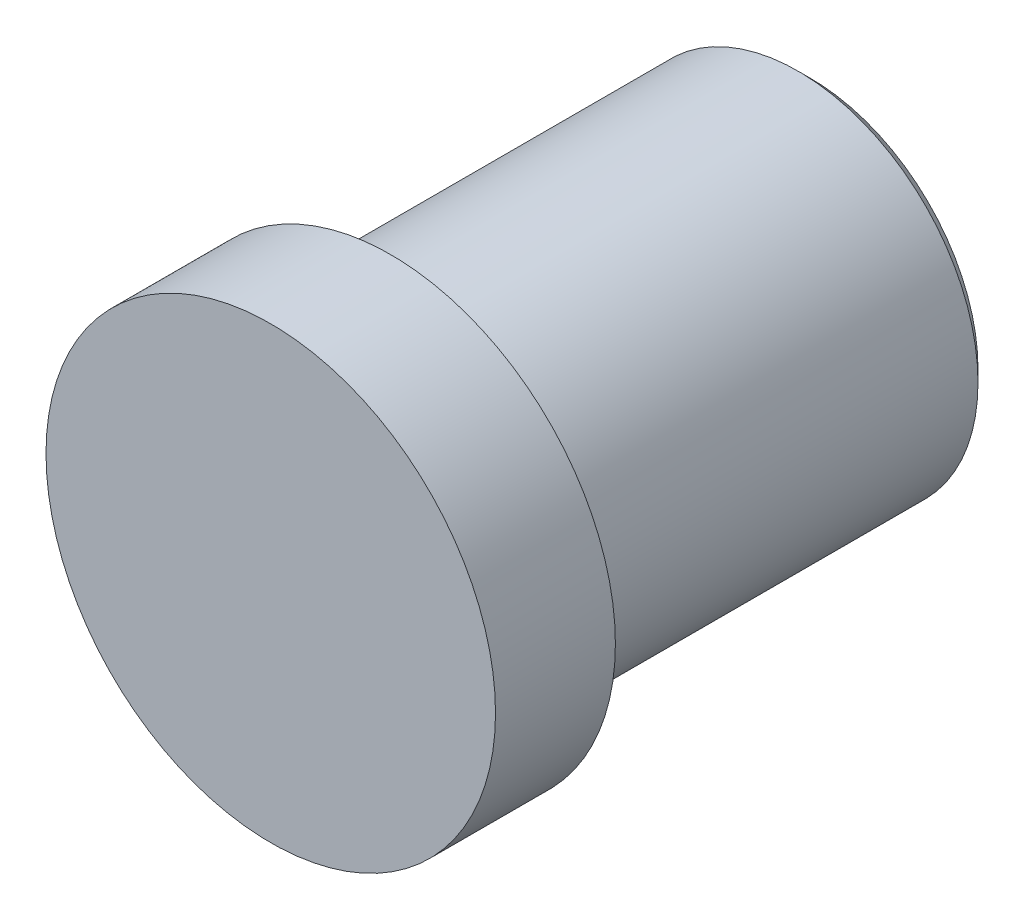
SolidWorks part; units mm, degrees
material "Q345"
ref_plane "前视基准面" through (0, 0, 0) normal (0, 0, 1) x (1, 0, 0)
ref_plane "上视基准面" through (0, 0, 0) normal (0, 1, 0) x (1, 0, 0)
ref_plane "右视基准面" through (0, 0, 0) normal (1, 0, 0) x (0, 0, -1)
sketch "草图1" plane through (0, 0, 0) normal (0, 0, 1) x (1, 0, 0)
  circle A0 centre (0, 0) radius 30
  circle A1 centre (0, 0) radius 20 construction
  dimension "D1" = 60
  dimension "D2" = 40
extrude "凸台-拉伸1" add sketch "草图1" along normal blind 70
sketch "草图2" plane through (0, 0, 70) normal (0, 0, 1) x (1, 0, 0)
  circle A0 centre (0, 0) radius 37.5
  dimension "D1" = 75
extrude "凸台-拉伸2" add sketch "草图2" along normal blind 20
chamfer "倒角2" distance 2 angle 45 1 edges at (30, 0, 0)
ref_axis "基准轴1" through (0, 0, 70) along (0, 0, -1)
sketch "草图3" plane through (0, 0, 0) normal (0, 1, 0) x (1, 0, 0)
  line L1 (30, -70) -> (29, -70)
  line L2 (30, -70) -> (30, -68)
  line L3 (30, -68) -> (29, -68)
  line L4 (29, -70) -> (29, -68)
  dimension "D1" = 2
  dimension "D2" = 1
revolve "切除-旋转1" cut sketch "草图3" angle 360 about axis through (0, 0, 70) along (0, 0, -1)
